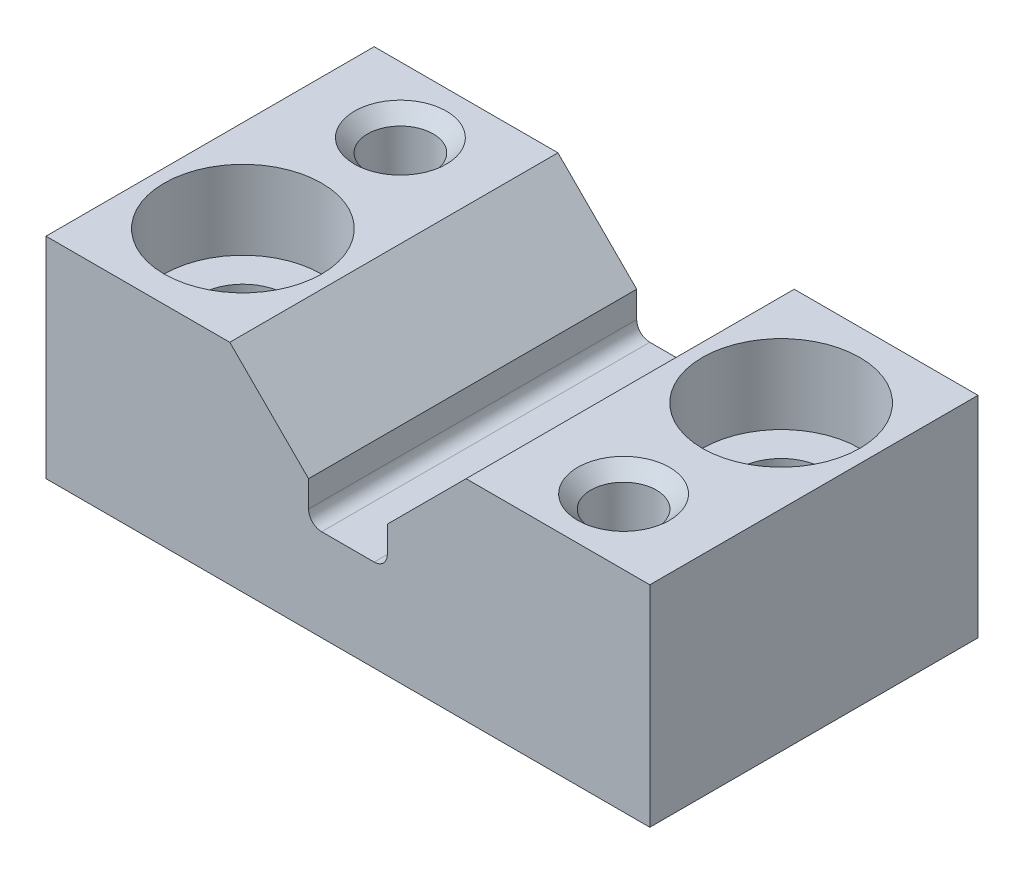
from build123d import *

# Parameters (mm, degrees)
SKETCH1_W          = 46
SKETCH1_H          = 16
BOSS_EXTRUDE_DEPTH = 25
CUT_EXTRUDE1_DEPTH = 38.549966711
SKETCH4_R          = 3.3
SKETCH4_R_2        = 2.5
CUT_EXTRUDE4_DEPTH = 38.549966711
FILLET1_R          = 1
FILLET2_R          = 1
SKETCH5_R          = 6
CUT_EXTRUDE5_DEPTH = 6
CHAMFER1_SIZE      = 1
CHAMFER2_SIZE      = 1
CHAMFER3_SIZE      = 1
CHAMFER4_SIZE      = 1


with BuildPart() as part:
    # Sketch1 → Boss-Extrude (new body)
    with BuildSketch(Plane.XY):
        with Locations((0, -8)):
            Rectangle(SKETCH1_W, SKETCH1_H)
    extrude(amount=BOSS_EXTRUDE_DEPTH)

    # Sketch2 → Cut-Extrude1 (cut, through all)
    with BuildSketch(Plane.XY.offset(25)):
        Polygon((-3, -9), (3, -9), (3, -6), (9, 0), (-9, 0), (-3, -6), align=None)
    extrude(amount=-CUT_EXTRUDE1_DEPTH, mode=Mode.SUBTRACT)

    # Sketch4 → Cut-Extrude4 (cut, through all)
    with BuildSketch(Plane(origin=(0, 0, 0), x_dir=(-1, 0, 0), z_dir=(0, 1, 0))):
        with Locations(Location((16, 17, 0), (0, 0, 90))):
            Circle(SKETCH4_R)
        with Locations(Location((16, 5, 0), (0, 0, 90))):
            Circle(SKETCH4_R_2)
        with Locations(Location((-16, 20, 0), (0, 0, 90))):
            Circle(SKETCH4_R_2)
        with Locations(Location((-16, 8, 0), (0, 0, 90))):
            Circle(SKETCH4_R)
    extrude(amount=-CUT_EXTRUDE4_DEPTH, mode=Mode.SUBTRACT)

    # Fillet1
    fillet1_edges = [part.edges().sort_by_distance(p)[0] for p in [
        (-3, -9, 12.5),
    ]]
    fillet(fillet1_edges, radius=FILLET1_R)

    # Fillet2
    fillet2_edges = [part.edges().sort_by_distance(p)[0] for p in [
        (3, -9, 12.5),
    ]]
    fillet(fillet2_edges, radius=FILLET2_R)

    # Sketch5 → Cut-Extrude5 (cut)
    with BuildSketch(Plane(origin=(0, 0, 0), x_dir=(-1, 0, 0), z_dir=(0, 1, 0))):
        with Locations(Location((16, 17, 0), (0, 0, 90))):
            Circle(SKETCH5_R)
        with Locations(Location((-16, 8, 0), (0, 0, 90))):
            Circle(SKETCH5_R)
    extrude(amount=-CUT_EXTRUDE5_DEPTH, mode=Mode.SUBTRACT)

    # Chamfer1
    chamfer1_edges = [part.edges().sort_by_distance(p)[0] for p in [
        (16, 0, 17.5),
    ]]
    chamfer(chamfer1_edges, length=CHAMFER1_SIZE)

    # Chamfer2
    chamfer2_edges = [part.edges().sort_by_distance(p)[0] for p in [
        (-16, 0, 2.5),
    ]]
    chamfer(chamfer2_edges, length=CHAMFER2_SIZE)

    # Chamfer3
    chamfer3_edges = [part.edges().sort_by_distance(p)[0] for p in [
        (16, -16, 17.5),
    ]]
    chamfer(chamfer3_edges, length=CHAMFER3_SIZE)

    # Chamfer4
    chamfer4_edges = [part.edges().sort_by_distance(p)[0] for p in [
        (-16, -16, 2.5),
    ]]
    chamfer(chamfer4_edges, length=CHAMFER4_SIZE)


solid = part.part
